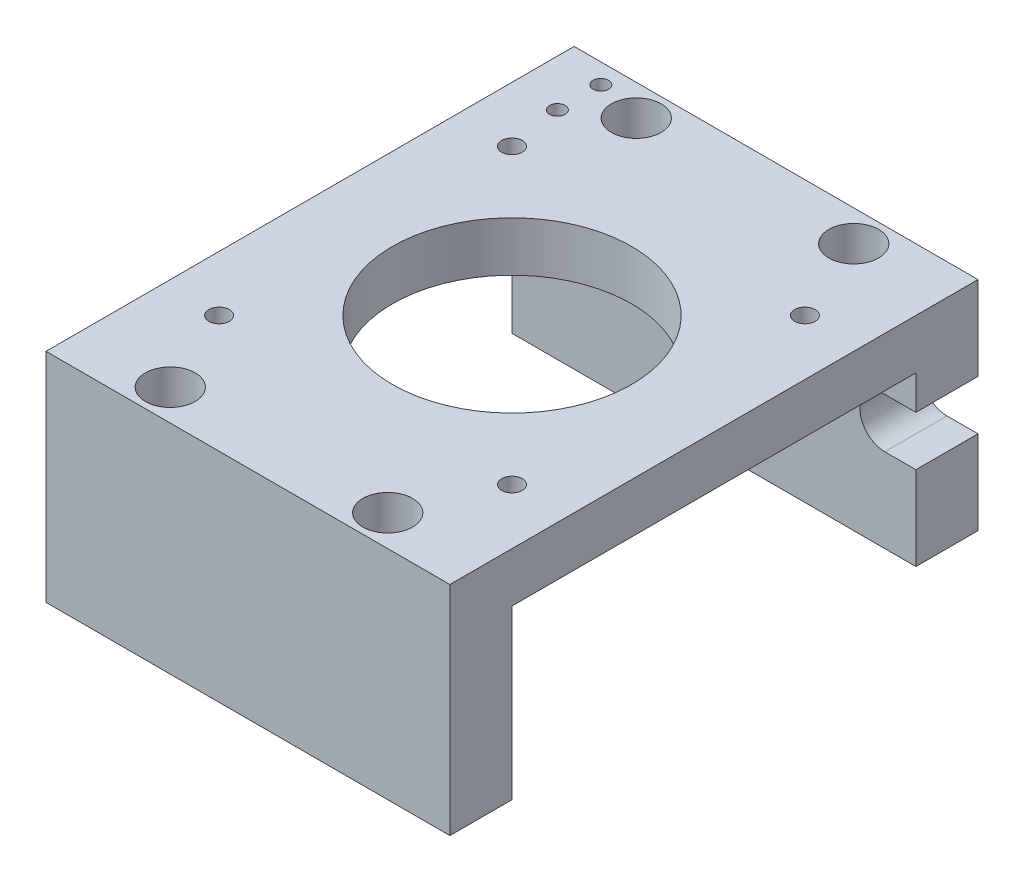
SolidWorks part; units mm, degrees
ref_plane "前视基准面" through (0, 0, 0) normal (0, 0, 1) x (1, 0, 0)
ref_plane "上视基准面" through (0, 0, 0) normal (0, 1, 0) x (1, 0, 0)
ref_plane "右视基准面" through (0, 0, 0) normal (1, 0, 0) x (0, 0, -1)
sketch "草图1" plane through (0, 0, 0) normal (0, 1, 0) x (1, 0, 0)
  line L1 (-32.5, 42.5) -> (32.5, 42.5)
  line L2 (-32.5, 42.5) -> (-32.5, -42.5)
  line L3 (-32.5, -42.5) -> (32.5, -42.5)
  line L4 (32.5, 42.5) -> (32.5, -42.5)
  line L5 (-32.5, 42.5) -> (32.5, -42.5) construction
  line L6 (-32.5, -42.5) -> (32.5, 42.5) construction
  point P0 (0, 0)
  dimension "D1" = 65
  dimension "D2" = 85
extrude "凸台-拉伸1" add sketch "草图1" along normal blind 35
sketch "草图2" plane through (0, 0, 0) normal (0, -1, 0) x (1, 0, 0)
  line L1 (-54.9857, 32.5) -> (54.9857, 32.5)
  line L2 (-54.9857, 32.5) -> (-54.9857, -32.5)
  line L3 (-54.9857, -32.5) -> (54.9857, -32.5)
  line L4 (54.9857, 32.5) -> (54.9857, -32.5)
  line L5 (-54.9857, 32.5) -> (54.9857, -32.5) construction
  line L6 (-54.9857, -32.5) -> (54.9857, 32.5) construction
  point P0 (0, 0)
  dimension "D1" = 65
extrude "切除-拉伸1" cut sketch "草图2" against normal offset from surface (27 mm away) 8 up to face at (0, 35, 0)
sketch "草图3" plane through (0, 35, 0) normal (0, 1, 0) x (1, 0, 0)
  circle A0 centre (0, 0) radius 19.25
  dimension "D1" = 38.5
extrude "切除-拉伸2" cut sketch "草图3" against normal through all
hole_wizard "M4 螺纹孔1" positions "草图5" profile "草图4" tap size "M4" standard "GB" end condition through all
sketch "草图5" plane through (0, 35, 0) normal (0, 1, 0) x (1, 0, 0)
  line L0 (-23.57, 23.57) -> (23.57, 23.57) construction
  line L1 (23.57, 23.57) -> (23.57, -23.57) construction
  line L4 (0, 0) -> (0, 23.57) construction
  line L7 (0, 0) -> (23.57, 0) construction
  point P0 (-23.57, 23.57)
  point P2 (23.57, 23.57)
  point P4 (-23.57, -23.57)
  point P6 (23.57, -23.57)
  dimension "D1" = 47.14
  dimension "D2" = 47.14
sketch "草图4" plane through (-23.57, 35, -23.57) normal (1, 0, 0) x (0, 0, 1)
  line L0 (0, 0) -> (0, 35)
  line L1 (0, 35) -> (1.65, 35)
  line L2 (1.65, 35) -> (1.65, 0)
  line L5 (1.65, 0) -> (0, 0)
  line L11 (0, -6.35) -> (0, 107.95) construction
  dimension "通孔螺纹孔钻头直径" = 3.3
  dimension "通孔螺纹孔钻头深度" = 35
cosmetic thread "孔螺蚊线1" parameters "D2"=4
cosmetic thread "孔螺蚊线2" parameters "D2"=4
cosmetic thread "孔螺蚊线3" parameters "D2"=4
cosmetic thread "孔螺蚊线4" parameters "D2"=4
hole_wizard "M3 螺纹孔1" positions "草图7" profile "草图6" tap size "M3" standard "GB"
sketch "草图7" plane through (-32.5, 0, 0) normal (-1, 0, 0) x (0, 0, 1)
  line L0 (-7.5, 31) -> (7.5, 31) construction
  line L3 (0, 31) -> (0, 0) construction
  line L6 (-42.5, 35) -> (42.5, 35) construction
  point P0 (7.5, 31)
  point P2 (-7.5, 31)
  dimension "D1" = 4
  dimension "D2" = 15
sketch "草图6" plane through (-32.5, 31, 7.5) normal (0, 1, 0) x (0, 0, 1)
  line L0 (0, 0) -> (0, 13.2511)
  line L1 (0, 13.2511) -> (1.25, 12.5)
  line L2 (1.25, 12.5) -> (1.25, 0)
  line L5 (1.25, 0) -> (0, 0)
  line L10 (0, 13.2511) -> (-1.25, 12.5) construction
  line L11 (0, -6.35) -> (0, 107.95) construction
  dimension "螺纹孔钻头直径" = 2.5
  dimension "螺纹孔钻头深度" = 12.5
  dimension "导头角度" = 118
cosmetic thread "孔螺蚊线5" parameters "D1"=10, "D2"=3
cosmetic thread "孔螺蚊线6" parameters "D1"=10, "D2"=3
hole_wizard "M3 螺纹孔2" positions "草图9" profile "草图8" tap size "M3" standard "GB"
sketch "草图9" plane through (0, 0, -42.5) normal (0, 0, -1) x (-1, 0, 0)
  line L2 (-32.5, 35) -> (32.5, 35) construction
  line L3 (-32.5, 35) -> (-32.5, 0) construction
  point P0 (-28.5, 12)
  point P2 (-28.5, 31)
  dimension "D1" = 4
  dimension "D2" = 19
  dimension "D3" = 4
sketch "草图8" plane through (28.5, 12, -42.5) normal (1, 0, 0) x (0, 1, 0)
  line L0 (0, 0) -> (0, 13.2511)
  line L1 (0, 13.2511) -> (1.25, 12.5)
  line L2 (1.25, 12.5) -> (1.25, 0)
  line L5 (1.25, 0) -> (0, 0)
  line L10 (0, 13.2511) -> (-1.25, 12.5) construction
  line L11 (0, -6.35) -> (0, 107.95) construction
  dimension "螺纹孔钻头直径" = 2.5
  dimension "螺纹孔钻头深度" = 12.5
  dimension "导头角度" = 118
cosmetic thread "孔螺蚊线7" [suppressed] parameters "D1"=10, "D2"=3
cosmetic thread "孔螺蚊线8" [suppressed] parameters "D1"=10, "D2"=3
sketch "草图10" plane through (0, 0, -42.5) normal (0, 0, -1) x (-1, 0, 0)
  line L0 (-27.5, 17.5) -> (-37.5, 17.5) construction
  line L2 (-27.5, 13.5) -> (-37.5, 13.5)
  line L3 (-27.5, 21.5) -> (-37.5, 21.5)
  line L4 (-32.5, 35) -> (-32.5, 0) construction
  arc A0 (-27.5, 13.5) -> (-27.5, 21.5) centre (-27.5, 17.5) ccw
  arc A1 (-37.5, 21.5) -> (-37.5, 13.5) centre (-37.5, 17.5) ccw
  point P4 (-32.5, 17.5)
  dimension "D1" = 5
  dimension "D2" = 8
extrude "切除-拉伸3" cut sketch "草图10" against normal blind 15
hole_wizard "打孔尺寸(%根据)开槽圆柱头螺钉的类型1" positions "草图12" profile "草图11" counterbore size "M4" standard "GB" end condition through all
sketch "草图12" plane through (0, 35, 0) normal (0, 1, 0) x (1, 0, 0)
  line L0 (-17.5, 37.5) -> (17.5, 37.5) construction
  line L1 (17.5, 37.5) -> (17.5, -37.5) construction
  line L4 (0, 0) -> (0, 37.5) construction
  line L7 (32.5, 0) -> (17.5, 0) construction
  line L8 (32.5, -42.5) -> (32.5, 42.5) construction
  line L11 (32.5, 42.5) -> (-32.5, 42.5) construction
  point P0 (-17.5, 37.5)
  point P2 (17.5, 37.5)
  point P4 (-17.5, -37.5)
  point P6 (17.5, -37.5)
  dimension "D1" = 35
  dimension "D2" = 5
sketch "草图11" plane through (-17.5, 35, -37.5) normal (1, 0, 0) x (0, 0, 1)
  line L0 (0, 0) -> (0, 35)
  line L1 (0, 35) -> (2.25, 35)
  line L3 (2.25, 35) -> (2.25, 20)
  line L4 (2.25, 20) -> (4, 20)
  line L5 (4, 20) -> (4, 0)
  line L7 (4, 0) -> (0, 0)
  line L11 (0, -6.35) -> (0, 107.95) construction
  dimension "通孔孔直径" = 4.5
  dimension "通孔孔深度" = 35
  dimension "柱形沉头孔直径" = 8
  dimension "柱形沉头孔深度" = 20
hole_wizard "M3 螺纹孔3" positions "草图13" profile "草图14" tap size "M3" standard "GB"
sketch "草图13" plane through (0, 35, 0) normal (0, 1, 0) x (1, 0, 0)
  point P0 (-25, 32.3)
  point P3 (-25, 39.3)
sketch "草图14" plane through (-25, 35, -32.3) normal (1, 0, 0) x (0, 0, 1)
  line L0 (0, 0) -> (0, 10.2511)
  line L1 (0, 10.2511) -> (1.25, 9.5)
  line L2 (1.25, 9.5) -> (1.25, 0)
  line L5 (1.25, 0) -> (0, 0)
  line L10 (0, 10.2511) -> (-1.25, 9.5) construction
  line L11 (0, -6.35) -> (0, 107.95) construction
  dimension "螺纹孔钻头直径" = 2.5
  dimension "螺纹孔钻头深度" = 9.5
  dimension "导头角度" = 118
cosmetic thread "孔螺蚊线9" parameters "D1"=8, "D2"=3
cosmetic thread "孔螺蚊线10" parameters "D1"=8, "D2"=3
